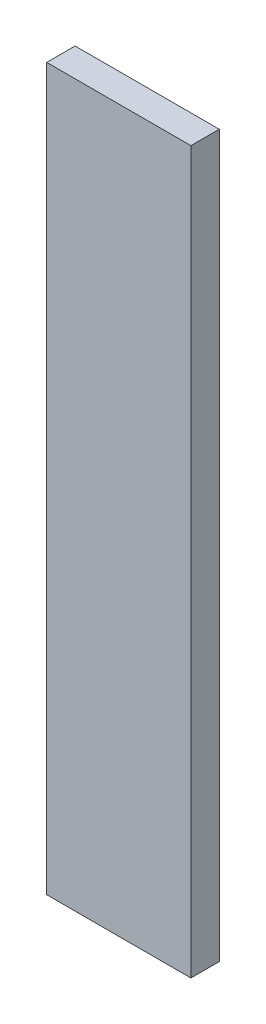
from build123d import *

# Parameters (mm, degrees)
SKETCH1_W           = 50.8
SKETCH1_H           = 254
BOSS_EXTRUDE1_DEPTH = 5


with BuildPart() as part:
    # Sketch1 → Boss-Extrude1 (new, symmetric)
    with BuildSketch(Plane.XY):
        Rectangle(SKETCH1_W, SKETCH1_H)
    extrude(amount=BOSS_EXTRUDE1_DEPTH, both=True)


solid = part.part
